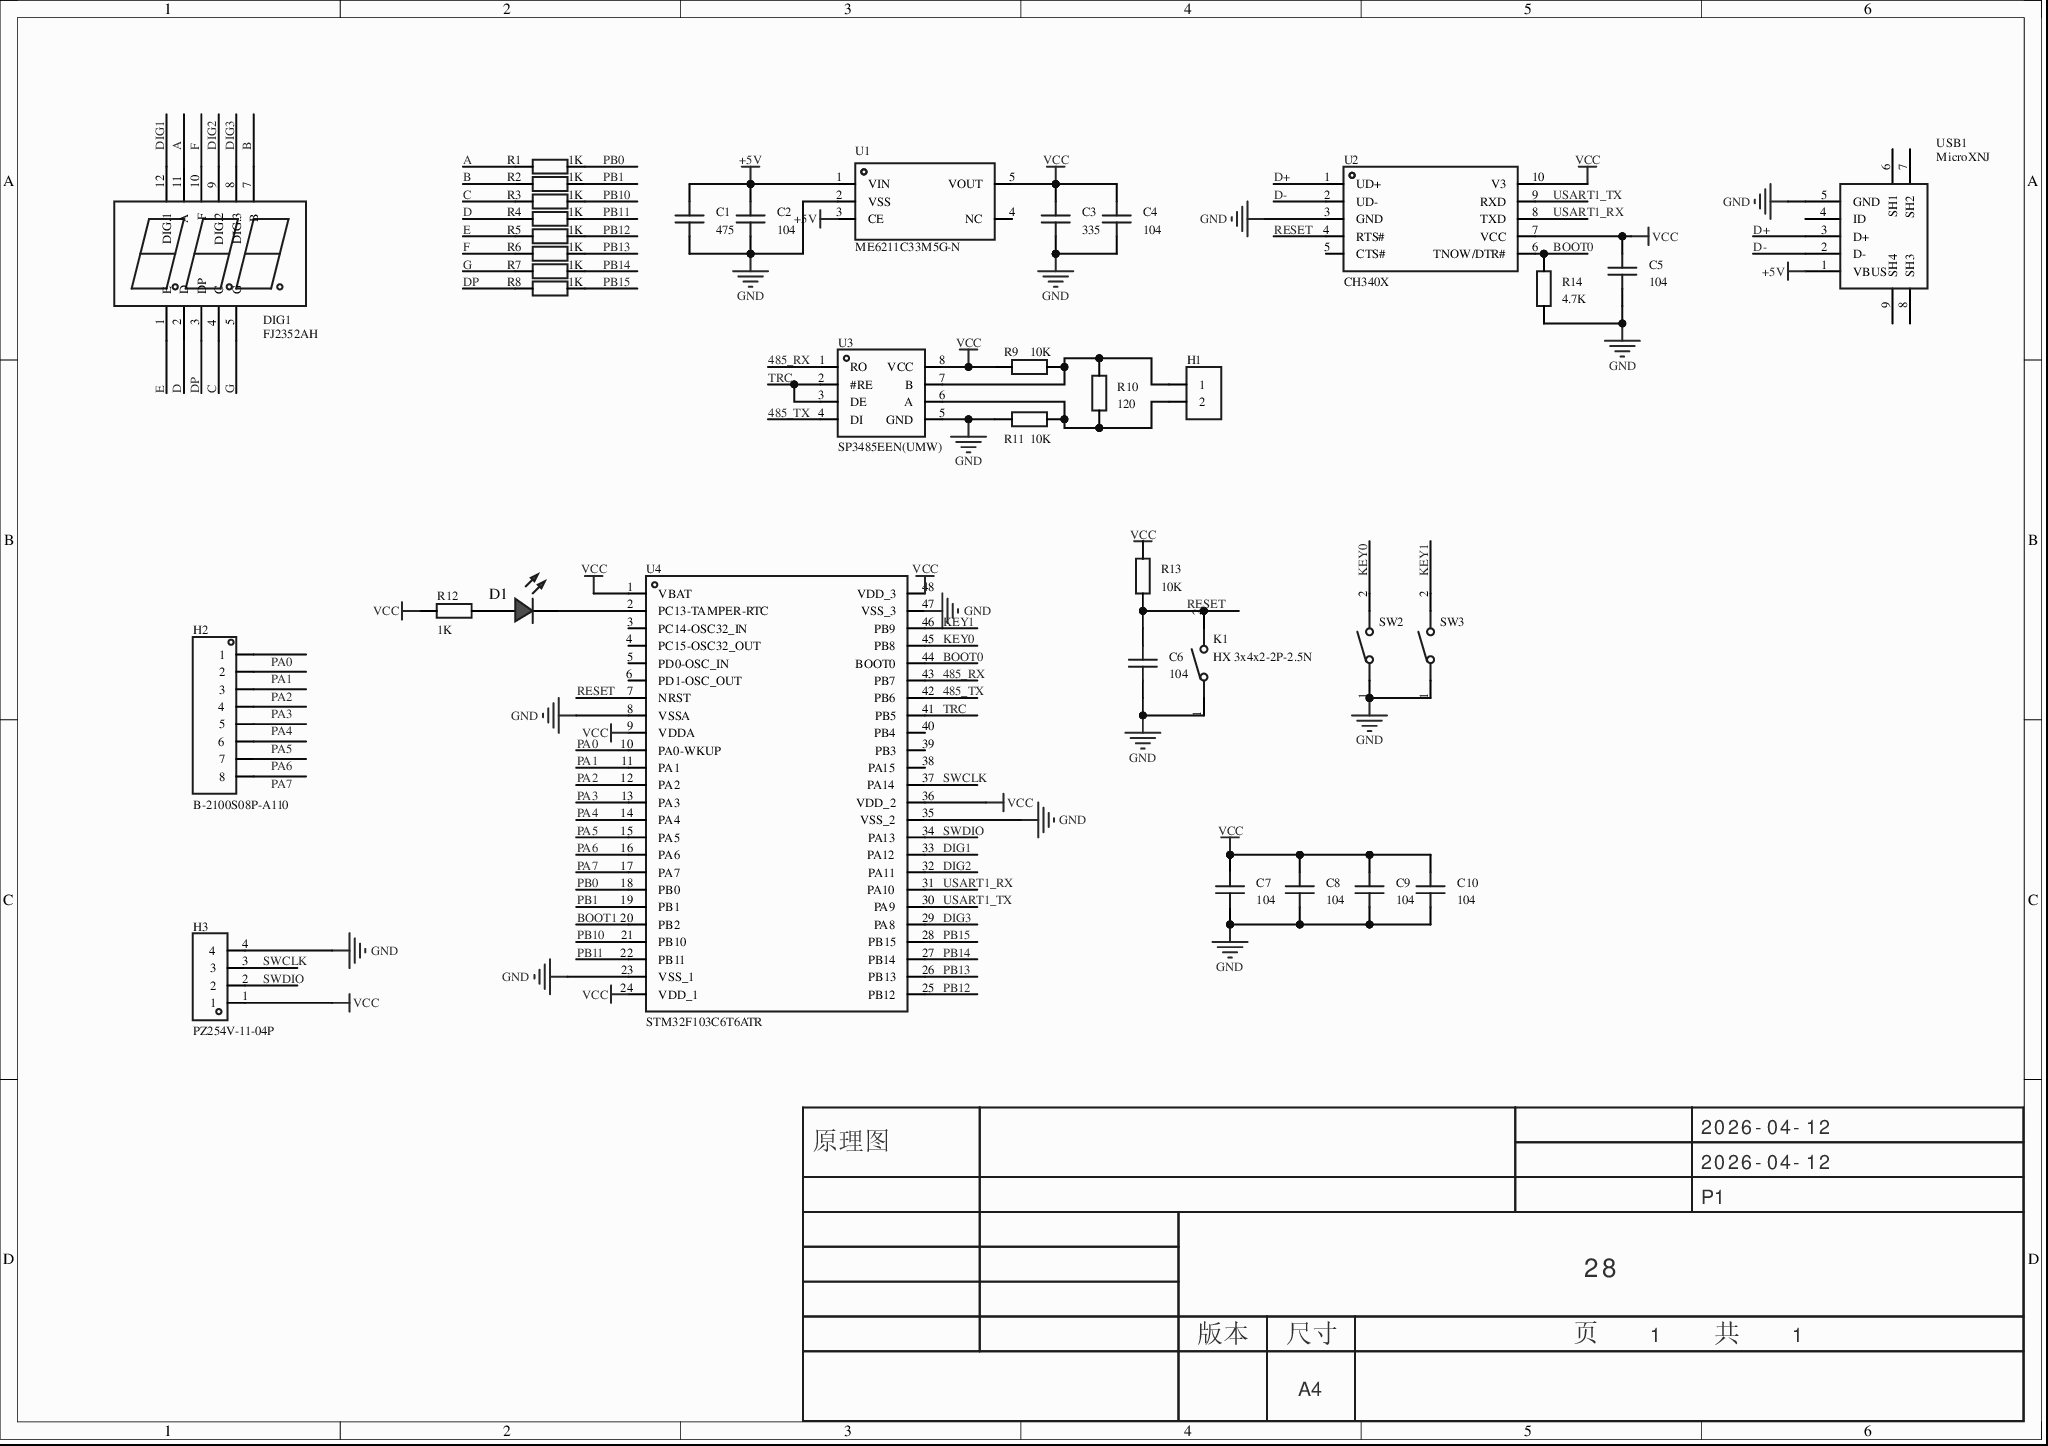
[diagram p0: MISC49919-3.schdoc]
# Altium project MISC49919-2.PrjPcb
1 sheet, 37 parts. Net scope: global (net labels, ports and power ports of the same name join across sheets).
Board file: MISC49919.pcbdoc

## Sheet MISC49919-3.schdoc
size 297 x 209 mm; Version: V1.0; @Project Name: MISC49919; @Update Date: 2026-04-12; @Create Date: 2026-04-12; @Board Name: MISC49919; @Create Time: 00:56:43; @Page Count: 1; @Page No: 1; @Schematic Name: MISC49919; @Update Time: 00:56:43; Size: A4

### Parts
C1  475  [C0805]
C2  104  [C0603]
C3  335  [C0805]
C4  104  [C0603]
C5  104  [C0603]
C6  104  [C0603]
C7  104  [C0603]
C8  104  [C0603]
C9  104  [C0603]
C10  104  [C0603]
D1  (no value)  [LED_0603]
DIG1  FJ2352AH  [LED-SEG-TH_FJ2352AH]
H1  (no value)  [HDR-TH_2P-P2.54-V-F]
H2  B-2100S08P-A110  [HDR-TH_8P-P2.54-V-M]
H3  PZ254V-11-04P  [HDR-TH_4P-P2.54-V-M]
K1  HX 3x4x2-2P-2.5N  [SW-SMD_L4.0-W2.9-LS5.0]
R1  1K  [R0603]
R2  1K  [R0603]
R3  1K  [R0603]
R4  1K  [R0603]
R5  1K  [R0603]
R6  1K  [R0603]
R7  1K  [R0603]
R8  1K  [R0603]
R9  10K  [R0603]
R10  120  [R0603]
R11  10K  [R0603]
R12  1K  [R0603]
R13  10K  [R0603]
R14  4.7K  [R0603]
SW2  HX 3x4x2-2P-2.5N  [SW-SMD_L4.0-W2.9-LS5.0]  (value not drawn)
SW3  HX 3x4x2-2P-2.5N  [SW-SMD_L4.0-W2.9-LS5.0]  (value not drawn)
U1  ME6211C33M5G-N  [SOT-23-5_L3.0-W1.7-P0.95-LS2.8-BL]
U2  CH340X  [MSOP-10_L3.0-W3.0-P0.50-LS5.0-BL]
U3  SP3485EEN(UMW)  [SOP-8_L5.0-W4.0-P1.27-LS6.0-BL]
U4  STM32F103C6T6ATR  [LQFP-48_L7.0-W7.0-P0.50-LS9.0-BL]
USB1  MicroXNJ  [MICRO-USB-SMD_MICROXNJ_1]

### Nets
+5V: C1.2 C2.2 U1.1(VIN) U1.3(CE) USB1.1(VBUS)
GND: C1.1 C2.1 C3.1 C4.1 C5.1 C6.1 C7.1 C8.1 C9.1 C10.1 H3.4 K1.1 R11.1 R14.1 SW2.1 SW3.1 U1.2(VSS) U2.3(GND) U3.5(GND) U4.8(VSSA) U4.23(VSS_1) U4.35(VSS_2) U4.47(VSS_3) USB1.5(GND)
VCC: C3.2 C4.2 C5.2 C7.2 C8.2 C9.2 C10.2 H3.1 R9.1 R12.1 R13.2 U1.5(VOUT) U2.7(VCC) U2.10(V3) U3.8(VCC) U4.1(VBAT) U4.9(VDDA) U4.24(VDD_1) U4.36(VDD_2) U4.48(VDD_3)
485_RX: U3.1(RO) U4.43(PB7)
485_TX: U3.4(DI) U4.42(PB6)
A: DIG1.11(A) R1.1
B: DIG1.7(B) R2.1
BOOT0: R14.2 U2.6(TNOW/DTR#) U4.44(BOOT0)
BOOT1: U4.20(PB2)
C: DIG1.4(C) R3.1
D: DIG1.2(D) R4.1
D+: U2.1(UD+) USB1.3(D+)
D-: U2.2(UD-) USB1.2(D-)
DIG1: DIG1.12(DIG.1) U4.33(PA12)
DIG2: DIG1.9(DIG.2) U4.32(PA11)
DIG3: DIG1.8(DIG.3) U4.29(PA8)
DP: DIG1.3(DP) R8.1
E: DIG1.1(E) R5.1
F: DIG1.10(F) R6.1
G: DIG1.5(G) R7.1
KEY0: SW2.2 U4.45(PB8)
KEY1: SW3.2 U4.46(PB9)
PA0: H2.1 U4.10(PA0-WKUP)
PA1: H2.2 U4.11(PA1)
PA2: H2.3 U4.12(PA2)
PA3: H2.4 U4.13(PA3)
PA4: H2.5 U4.14(PA4)
PA5: H2.6 U4.15(PA5)
PA6: H2.7 U4.16(PA6)
PA7: H2.8 U4.17(PA7)
PB0: R1.2 U4.18(PB0)
PB1: R2.2 U4.19(PB1)
PB10: R3.2 U4.21(PB10)
PB11: R4.2 U4.22(PB11)
PB12: R5.2 U4.25(PB12)
PB13: R6.2 U4.26(PB13)
PB14: R7.2 U4.27(PB14)
PB15: R8.2 U4.28(PB15)
RESET: C6.2 K1.2 R13.1 U2.4(RTS#) U4.7(NRST)
SWCLK: H3.3 U4.37(PA14)
SWDIO: H3.2 U4.34(PA13)
TRC: U3.2(#RE) U3.3(DE) U4.41(PB5)
USART1_RX: U2.8(TXD) U4.31(PA10)
USART1_TX: U2.9(RXD) U4.30(PA9)
NetD1_1: D1.1(C) U4.2(PC13-TAMPER-RTC)
NetD1_2: D1.2(A) R12.2
NetH1_1: H1.1 R9.2 R10.2 U3.7(B)
NetH1_2: H1.2 R10.1 R11.2 U3.6(A)

Not connected (* = marked no-connect by the designer): U1 4(NC); U2 5(CTS#)*; U4 3(PC14-OSC32_IN)* 4(PC15-OSC32_OUT)* 5(PD0-OSC_IN)* 6(PD1-OSC_OUT)* 38(PA15)* 39(PB3)* 40(PB4)*; USB1 4(ID)* 6(SH1)* 7(SH2)* 8(SH3)* 9(SH4)*

### Notes on the sheet
- 2026-04-12
- 原理图
- P1
- 28
- 版本
- 尺寸
- A4
- 页    1    共    1

### Library data of the parts
C1 C3 = CAP_0805: Symbol: Capacitance; ConvertToPcb: yes; ModelId: 1ba041120af144c991958decab20d2410819f05c4eef4c71ace90d822a990e87; ModelName: C0805_L2.0-W1.3-H1.3; ModelTransform: 78.74,51.181,0,0,0,0,0,0.0005,0; Device: CAP_0805; AddInBom: yes; Supplier Footprint: 0805; FootprintName: C0805
  C1: Value: 475
  C3: Value: 335
C2 C4-C10 = CAP_0603: Symbol: Capacitance; ConvertToPcb: yes; ModelId: ac125912035d415993ca9572d50418b10819f05c4eef4c71ace90d822a990e87; ModelName: C0603_L1.6-W0.8-H0.8; ModelTransform: 62.992,31.496,0,0,0,0,0,0,0; Device: CAP_0603; Value: 104; AddInBom: yes; Supplier Footprint: 0603; FootprintName: C0603
D1 = LED_0603-R: Symbol: LED_R; Convert to PCB: yes; 3D Model: dd8257b0d61a4cd7b68939a056e080950819f05c4eef4c71ace90d822a990e87; 3D Model Transform: 58.72,29.4,22.03,0,0,0,0,0,0; ModelName: LED-0603_R; Device: LED_0603-R; Add into BOM: yes; Supplier Footprint: 0603; FootprintName: LED_0603
DIG1 = FJ2352AH: 数码管位数:3位;字符尺寸(英寸):0.25;发光颜色:红色;LED极性:共阴极;; Manufacturer: 志浩; AddInBom: yes; ModelId: 5af869523f65472c910c1cc8f20b41320819f05c4eef4c71ace90d822a990e87; ModelTransform: 602.361,323.2277,0,0,0,0,0,0,-157.48; Number of Characters: 3位; Digit/Alpha Size(inch): 0.25; Illumination Color: 红色; LED Polarity: 共阴极; Symbol: FJ2352AH; Device: FJ2352AH; LCSC Part Name: 3位0.25英寸 共阴红光 数码管; SupplierPart: C2938365; ManufacturerPart: FJ2352AH; Supplier Footprint: 插件; JLCPCB Part Class: Extended Part; Datasheet: https://item.szlcsc.com/datasheet/FJ2352AH/3294654.html; Supplier: LCSC; ConvertToPcb: yes; FootprintName: LED-SEG-TH_FJ2352AH; ModelName: LED-SEG-TH_FJ2352AH
H1 = HDR-F_2.54_1x2P: Symbol: Header-Female-2.54_1x2; ConvertToPcb: yes; ModelId: a9450ef445564560a104363b9aacde4e0819f05c4eef4c71ace90d822a990e87; ModelName: HDR-TH_2P-P2.54-F-LI-1X2P; ModelTransform: 215.7476,98.425,0,0,0,0,0,0,-129.921; Device: HDR-F_2.54_1x2P; AddInBom: yes; SupplierPart: C49661; Supplier Footprint: 插件; FootprintName: HDR-TH_2P-P2.54-V-F
H2 = B-2100S08P-A110: 插针结构:1x8P;间距:2.54mm;行距:-;圆针/方针:方针;安装方式:直插;排数:单排;总PIN位数:8P;额定电流:3A;额定电压:-;配合针长度:6mm;塑高:2.54mm;端接针长度:3mm;触头材质:黄铜;触头镀层:-;工作温度:-40℃~+105℃;颜色:黑色;; Manufacturer: Ckmtw(灿科盟); Symbol: Header-Male-2.54_1x8; AddInBom: yes; ModelId: f5b96e27511e49e38545e53df23202020819f05c4eef4c71ace90d822a990e87; ModelTransform: 807.87244,98.425,0,0,0,0,0,0,-118.11; Pin Structure: 1x8P; Pitch: 2.54mm; Circluar Pins/Square Pins: 方针; Current Rating: 3A; Device: B-2100S08P-A110; LCSC Part Name: 1x8P 间距:2.54mm 方针 直插; SupplierPart: C124381; ManufacturerPart: B-2100S08P-A110; Supplier Footprint: 插件,P=2.54mm; JLCPCB Part Class: Extended Part; Datasheet: https://item.szlcsc.com/datasheet/B-2100S08P-A110/125656.html; Supplier: LCSC; ConvertToPcb: yes; FootprintName: HDR-TH_8P-P2.54-V-M; ModelName: HDR-TH_8P-P2.54-V-M; Row Spacing: -; Mounting Type: 直插; Number of Rows: 单排; Number of Pins: 8P; Voltage Rating (Max): -; Length of Mating Pin: 6mm; Insulation Height: 2.54mm; Length of End Connection Pin: 3mm; Contact Material: 黄铜; Contact Plating: -; Operating Temperature: -40℃~+105℃; Color: 黑色
H3 = PZ254V-11-04P_C492403: 插针结构:1x4P;间距:2.54mm;行距:-;圆针/方针:方针;安装方式:直插;排数:单排;总PIN位数:4P;额定电流:3A;额定电压:250V;配合针长度:6mm;塑高:2.5mm;端接针长度:3mm;触头材质:黄铜;触头镀层:-;工作温度:-40℃~+105℃;颜色:黑色;; Manufacturer: XFCN(兴飞); AddInBom: yes; ModelId: 112f4d05e8d64e99ab9a333894bea4f90819f05c4eef4c71ace90d822a990e87; ModelName: HDR-TH_4P-P2.54-M-LI-1X4P; ModelTransform: 399.999,104.7242,0,0,0,0,0,0,-118.11; Pin Structure: 1x4P; Pitch: 2.54mm; Circluar Pins/Square Pins: 方针; Current Rating: 3A; Voltage Rating (Max): 250V; Symbol: PZ254V-11-04P; Device: PZ254V-11-04P_C492403; LCSC Part Name: 1x4P 间距:2.54mm 方针 直插; SupplierPart: C492403; ManufacturerPart: PZ254V-11-04P; Supplier Footprint: 插件,P=2.54mm; JLCPCB Part Class: Extended Part; Datasheet: https://item.szlcsc.com/datasheet/PZ254V-11-04P/502959.html; Supplier: LCSC; ConvertToPcb: yes; FootprintName: HDR-TH_4P-P2.54-V-M; Row Spacing: -; Mounting Type: 直插; Number of Rows: 单排; Number of Pins: 4P; Length of Mating Pin: 6mm; Insulation Height: 2.5mm; Length of End Connection Pin: 3mm; Contact Material: 黄铜; Contact Plating: -; Operating Temperature: -40℃~+105℃; Color: 黑色
K1 SW2 SW3 = HX 3x4x2-2P-2.5N: 电路结构:单刀单掷;按钮形状:圆形按钮;作用力:2.5N;安装方式:立贴;开关长度:4mm;开关宽度:3mm;开关高度:2mm;带支架:不带支架;触点电流:50mA;额定电压:12V;带灯:无;工作寿命:10万次;; Manufacturer: hanxia(韩下); Symbol: HX TS-1088-AR02016; AddInBom: yes; ModelId: 63599cce708d48afbce1b0db003544770819f05c4eef4c71ace90d822a990e87; ModelName: SW-SMD_L4.0-W2.9-H2-LS5.0; ModelTransform: 196.85,114.173,0,0,0,0,0,0,0; Circuit: 单刀单掷; Actuator Style: 圆形按钮; Operating Force: 2.5N; Switch Height: 2mm; with Bracket: 不带支架; Contact Current: 50mA; Voltage Rating: 12V; Actuator/Cap Color: 黑色; With Lamp: 无; Life: 10万次; Device: HX 3x4x2-2P-2.5N; LCSC Part Name: 4*3*2mm 立贴 轻触开关; SupplierPart: C36498961; ManufacturerPart: HX 3x4x2-2P-2.5N; Supplier Footprint: SMD,3x4mm; JLCPCB Part Class: Extended Part; Datasheet: https://item.szlcsc.com/datasheet/HX%25203x4x2-2P-2.5N/38220903.html; Supplier: LCSC; ConvertToPcb: yes; FootprintName: SW-SMD_L4.0-W2.9-LS5.0; Mounting Type: 立贴; Length: 4mm; Width: 3mm; IP Rating: -; Termination Style: SMD接片; Operating Temperature: -
R1-R9 R11-R14 = Res_0603: Symbol: 电阻; ConvertToPcb: yes; ModelId: fc143cca1e79419f9cd78b61e9279f080819f05c4eef4c71ace90d822a990e87; ModelTransform: 31.8897,63.7794,0,90,0,0,0,0,0; Device: Res_0603; AddInBom: yes; Supplier Footprint: 0603; FootprintName: R0603; ModelName: R0603
  R1-R8 R12: Value: 1K
  R9 R11 R13: Value: 10K
  R14: Value: 4.7K
R10 = Res_0603: Symbol: 电阻; 3D Model: fc143cca1e79419f9cd78b61e9279f080819f05c4eef4c71ace90d822a990e87; 3D Model Transform: 31.8897,63.7794,0,90,0,0,0,0,0; ConvertToPcb: yes; Device: Res_0603; Value: 120; Supplier Footprint: 0603; AddInBom: yes; FootprintName: R0603; ModelName: R0603
U1 = ME6211C33M5G-N: 输出类型:固定;工作电压:6V;输出电压:3.3V;输出电流:500mA;电源纹波抑制比(PSRR):70dB@(1kHz);输出极性:正极;; Manufacturer: MICRONE(南京微盟); AddInBom: yes; ModelId: 0a2a1b8f50944f73965918ad6e5fe1670819f05c4eef4c71ace90d822a990e87; ModelName: SOT-23-5_L2.9-W1.6-H1.1-LS2.8-P0.95; ModelTransform: 118.60433,114.173,0,90,0,0,0.0005,0.0005,0; Output Type: 固定; Voltage - Supply: 6V; Output Voltage: 3.3V; Output Current: 500mA; Voltage Dropout: 120mV@(100mA); standby current: 60uA; Noise: 50uVrms; Output Configuration: 正极; Number of Outputs: 1; Symbol: ME6211C33M5G-N; Device: ME6211C33M5G-N; LCSC Part Name: 输入6V 输出3.3V 500mA; SupplierPart: C82942; ManufacturerPart: ME6211C33M5G-N; Supplier Footprint: SOT-23-5; JLCPCB Part Class: Extended Part; Datasheet: https://item.szlcsc.com/datasheet/ME6211C33M5G-N/84106.html; Supplier: LCSC; ConvertToPcb: yes; FootprintName: SOT-23-5_L3.0-W1.7-P0.95-LS2.8-BL; Power Supply Rejection Ratio (PSRR): 70dB@(1kHz); Features: 过流保护；带使能；短路保护; Operating Temperature: -40℃~+150℃
U2 = CH340X: 应用功能:USB转串口；USB转并口;USB协议版本:USB 2.0;通道数:-;数据速率:2Mbps;; Manufacturer: WCH(南京沁恒); AddInBom: yes; ModelId: b42a31f9e1fa4643bc7ea573b9bba7ed0819f05c4eef4c71ace90d822a990e87; ModelName: MSOP-10_L3.0-W3.0-H1.1-LS5.0-P0.50; ModelTransform: 118.11,196.85,0,0,0,0,0,0,0; USB Protocol: USB 2.0; Voltage - Supply: 3.3V；5V; Data Rate: 2Mbps; Symbol: CH340X; Device: CH340X; LCSC Part Name: CH340X; SupplierPart: C3035748; ManufacturerPart: CH340X; Supplier Footprint: MSOP-10; JLCPCB Part Class: Extended Part; Datasheet: https://item.szlcsc.com/datasheet/CH340X/3584030.html; Supplier: LCSC; ConvertToPcb: yes; FootprintName: MSOP-10_L3.0-W3.0-P0.50-LS5.0-BL; Applications Function: USB转串口；USB转并口; Number of Channels: -; Operating Temperature: -20℃~+70℃; Current - Supply: -; Quiescent Supply Current: -
U3 = SP3485EEN(UMW): 类型:收发器;数据速率:12Mbps;; Manufacturer: UMW(友台半导体); AddInBom: yes; ModelId: a3315c1c78f949e6bb82c6eaca1c53c70819f05c4eef4c71ace90d822a990e87; ModelName: SOP-8_L5.0-W4.0-H1.8-LS6.2-P1.27; ModelTransform: 244.094,196.85,0,90,0,0,0,0,0; Number of Drivers: 1; Voltage - Supply: 2.97V~3.63V; Data Rate: 12Mbps; Number of Nodes: 256; Supply Current (Iq): 520uA; Communication Mode: 半双工; Symbol: SP3485EEN; Device: SP3485EEN(UMW); LCSC Part Name: SP3485E 3.3V电源，最多256个节点，12Mbps半双工，RS485/RS422收发器; SupplierPart: C668205; ManufacturerPart: SP3485EEN(UMW); Supplier Footprint: SOP-8; JLCPCB Part Class: Extended Part; Datasheet: https://item.szlcsc.com/datasheet/SP3485EEN(UMW)/698053.html; Supplier: LCSC; ConvertToPcb: yes; FootprintName: SOP-8_L5.0-W4.0-P1.27-LS6.0-BL; Type: 收发器; Number of Receivers: 1; Operating Temperature: -40℃~+85℃
U4 = STM32F103C6T6ATR: CPU内核:ARM-M3;CPU最大主频:72MHz;应用领域:-;; Manufacturer: ST(意法半导体); AddInBom: yes; ModelId: 093be70396ff421eb2cdb946d5311efc0819f05c4eef4c71ace90d822a990e87; ModelName: LQFP-48_L7.0-W7.0-H1.4-LS9.0-P0.50; ModelTransform: 354.331,354.331,0,0,0,0,0,0,0; CPU Core: ARM-M3; CPU Maximum Speed: 72MHz; Program Storage Size: 32KB; Program Memory Type: FLASH; Number of I/O: 37; ADC (Bit): 12bit; Voltage - Supply: 2V~3.6V; Symbol: STM32F103C6T6ATR; Device: STM32F103C6T6ATR; LCSC Part Name: 主流增强型ARM Cortex-M3 MCU，具有32 KB Flash、72 MHz CPU、电机控制、USB和CAN; SupplierPart: C2053946; ManufacturerPart: STM32F103C6T6ATR; Supplier Footprint: LQFP-48(7x7); JLCPCB Part Class: Extended Part; Datasheet: https://item.szlcsc.com/datasheet/STM32F103C6T6ATR/2145518.html; Supplier: LCSC; ConvertToPcb: yes; FootprintName: LQFP-48_L7.0-W7.0-P0.50-LS9.0-BL; Applications: -
USB1 = MicroXNJ: 连接器类型:Micro-B;协议标准:USB 2.0;公母:母;安装方式:卧贴;触点数量:5P;端口数量:1;额定电流 - 电源:1.8A;工作温度:-20℃~+85℃;; Manufacturer: SHOU HAN(首韩); AddInBom: yes; ModelId: d71825624ed74c65b7c976fd09fd0f0f0819f05c4eef4c71ace90d822a990e87; ModelTransform: 314.96,234.80992,0,0,0,0,0,-44.094,-35.433; Protocol Standard: USB 2.0; Gender: 母; Number of Contacts: 5P; Number of Ports: 1; Current Rating-Power: 1.8A; Voltage Rating: 30V; Connect-Disconnect Life: 5千次; Detection color: 黑色; Symbol: MICROXNJ; Device: MicroXNJ; LCSC Part Name: Micro小牛角卧贴母座; SupplierPart: C404969; ManufacturerPart: MicroXNJ; Supplier Footprint: SMD; JLCPCB Part Class: Extended Part; Datasheet: https://item.szlcsc.com/datasheet/MicroXNJ/392534.html; Supplier: LCSC; ConvertToPcb: yes; FootprintName: MICRO-USB-SMD_MICROXNJ_1; ModelName: MICRO-USB-SMD_MICROXNJ_1; Connector Type: Micro-B; Mounting Type: 卧贴; Operating Temperature: -20℃~+85℃